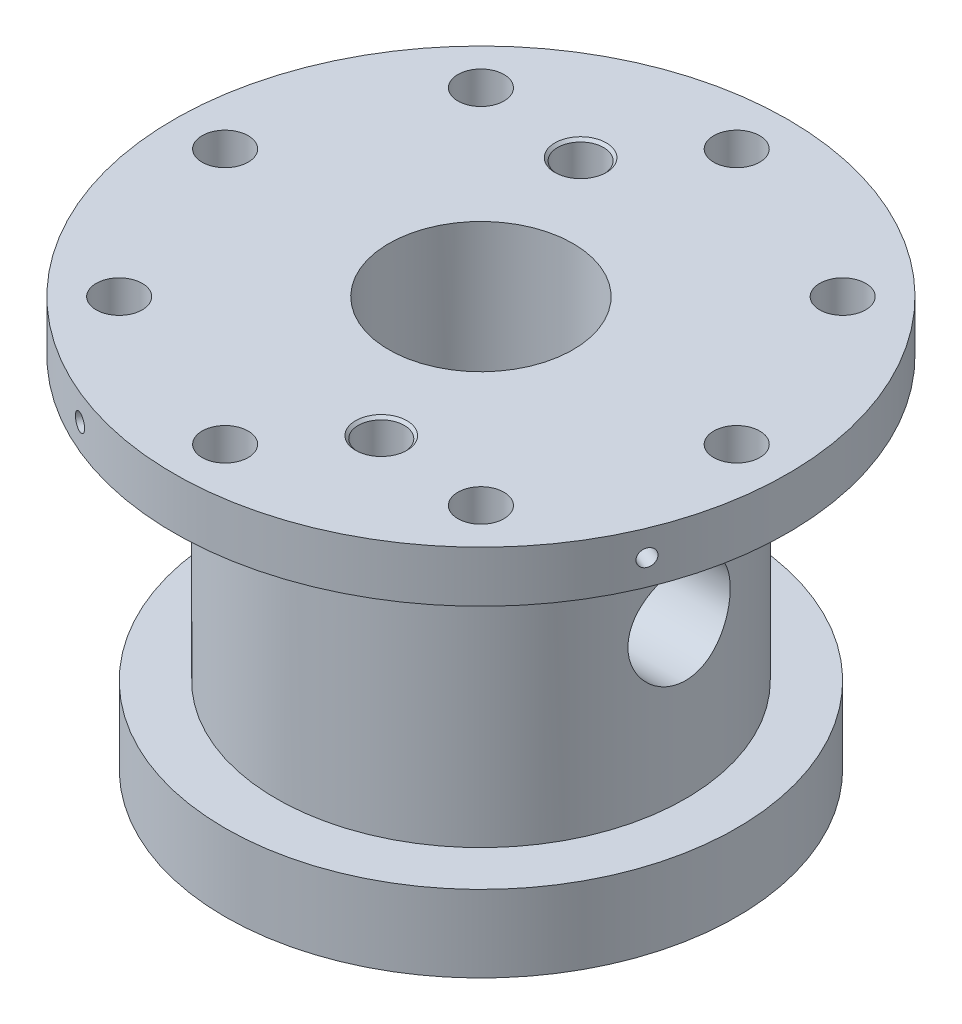
from build123d import *

# Parameters (mm, degrees)
SKETCH_2_R               = 4.5
CUT_EXTRUDE_1_DEPTH      = 10
PATTERN_CIRCULAR_1_COUNT = 8
EXTRUDE_START            = 10
SKETCH_3_R               = 40
EXTRUDE_1_DEPTH          = 10
SKETCH_7_R               = 18
EXTRUDE_2_DEPTH          = 10
SKETCH_5_W               = 5
SKETCH_5_H               = 30
CUT_EXTRUDE_2_DEPTH      = 15
PATTERN_CIRCULAR_3_COUNT = 3
PATTERN_CIRCULAR_4_COUNT = 4
EXTRUDE_3_DEPTH          = 10
EXTRUDE_3_DEPTH_BACK     = 5
SKETCH_11_R              = 50
SKETCH_11_W              = 5
SKETCH_11_H              = 30
M10X1_0_1_D              = 9
M10X1_0_1_DEPTH          = 23
M10X1_0_1_CSINK_D        = 10.05
M10X1_0_1_CSINK_ANGLE    = 90
M10X1_0_1_TIP            = 2.703872786
SKETCH_16_R              = 10
CUT_EXTRUDE_3_DEPTH      = 65


with BuildPart() as part:
    # 草图1 → 旋转1 (revolve)
    with BuildSketch(Plane.XY, mode=Mode.PRIVATE) as revolve_1_sk:
        Polygon((18, 60), (60, 60), (60, 50), (40, 50), (40, 0), (18, 0), align=None)
    revolve(revolve_1_sk.sketch.rotate(Axis((0, 0, 0), (0, 1, 0)), 90), axis=Axis((0, 0, 0), (0, 1, 0)))

    # 草图2 → 切除-拉伸1 (cut)
    with BuildSketch(Plane(origin=(0, 60, 0), x_dir=(1, 0, 0), z_dir=(0, 1, 0))):
        with Locations(Location((0, 50, 0), (0, 0, 270))):
            Circle(SKETCH_2_R)
    cut_extrude_1 = extrude(amount=-CUT_EXTRUDE_1_DEPTH, mode=Mode.SUBTRACT)

    # 阵列(圆周)1: 切除-拉伸1 ×8 about axis
    pattern_circular_1_axis = Axis((0, 0, 0), (0, 1, 0))
    for i in range(1, PATTERN_CIRCULAR_1_COUNT):
        add(cut_extrude_1.rotate(pattern_circular_1_axis, i * 360 / PATTERN_CIRCULAR_1_COUNT), mode=Mode.SUBTRACT)

    # 草图3 → 凸台-拉伸1 (add)
    with BuildSketch(Plane.XZ.offset(EXTRUDE_START)):
        with Locations(Location((0, 0, 0), (0, 0, 270))):
            Circle(SKETCH_3_R)
    extrude(amount=-EXTRUDE_1_DEPTH)

    # 草图7 → 凸台-拉伸2 (add)
    with BuildSketch(Plane(origin=(0, 0, 0), x_dir=(1, 0, 0), z_dir=(0, 1, 0)).offset(EXTRUDE_START)):
        with Locations(Location((0, 0, 0), (0, 0, 90))):
            Circle(SKETCH_7_R)
    extrude(amount=-EXTRUDE_2_DEPTH)

    # 草图5 → 切除-拉伸2 (cut)
    with BuildSketch(Plane.XZ.offset(10)):
        with Locations((0, 22)):
            Rectangle(SKETCH_5_W, SKETCH_5_H)
    cut_extrude_2 = extrude(amount=-CUT_EXTRUDE_2_DEPTH, mode=Mode.SUBTRACT)

    # 阵列(圆周)3: 切除-拉伸2 ×3 about axis
    pattern_circular_3_axis = Axis((0, 0, 0), (0, 1, 0))
    for i in range(1, PATTERN_CIRCULAR_3_COUNT):
        add(cut_extrude_2.rotate(pattern_circular_3_axis, i * 360 / PATTERN_CIRCULAR_3_COUNT), mode=Mode.SUBTRACT)

    # 草图10 → M4x0.7 螺纹孔1 (revolve, cut)
    with BuildSketch(Plane(origin=(22.961005942, 55, -55.432771951), x_dir=(-0.9238795325112892, 0, -0.3826834323650839), z_dir=(0, 1, 0))):
        Polygon((0, 0), (0, 11.091420021), (1.65, 10.1), (1.65, 0), align=None)
    m4x0_7_1 = revolve(axis=Axis((25.391045737, 55, -61.299406982), (-0.3826834323650839, 0, 0.9238795325112892)), mode=Mode.SUBTRACT)

    # 阵列(圆周)4: M4x0.7 螺纹孔1 ×4 about axis
    pattern_circular_4_axis = Axis((0, 0, 0), (0, -1, 0))
    for i in range(1, PATTERN_CIRCULAR_4_COUNT):
        add(m4x0_7_1.rotate(pattern_circular_4_axis, i * 360 / PATTERN_CIRCULAR_4_COUNT), mode=Mode.SUBTRACT)

    # 草图11 → 凸台-拉伸3 (add, two sides: drawn at the far end of the back side and taken through both)
    with BuildSketch(Plane.XZ.offset(10).offset(-EXTRUDE_3_DEPTH_BACK)):
        with Locations(Location((0, 0, 0), (0, 0, 270))):
            Circle(SKETCH_11_R)
        with Locations((0, 22)):
            Rectangle(SKETCH_11_W, SKETCH_11_H, mode=Mode.SUBTRACT)
        Polygon((-4.812177826, -5.665063509), (-30.79293994, -20.665063509), (-33.29293994, -16.334936491), (-7.312177826, -1.334936491), align=None, mode=Mode.SUBTRACT)
        Polygon((7.312177826, -1.334936491), (33.29293994, -16.334936491), (30.79293994, -20.665063509), (4.812177826, -5.665063509), align=None, mode=Mode.SUBTRACT)
    extrude(amount=EXTRUDE_3_DEPTH + EXTRUDE_3_DEPTH_BACK)

    # M10x1.0 螺纹孔1
    with Locations(Plane(origin=(-13.776603565, 60, -33.25966317), x_dir=(0, 0, 1), z_dir=(0, 1, 0))):
        with Locations((0, 0), (66.51932634, 27.55320713)):
            CounterSinkHole(M10X1_0_1_D / 2, M10X1_0_1_CSINK_D / 2, depth=M10X1_0_1_DEPTH, counter_sink_angle=M10X1_0_1_CSINK_ANGLE)
            with Locations((0, 0, -(M10X1_0_1_DEPTH + M10X1_0_1_TIP / 2))):  # 118° drill point
                Cone(0, M10X1_0_1_D / 2, M10X1_0_1_TIP, mode=Mode.SUBTRACT)

    # 草图16 → 切除-拉伸3 (cut, symmetric)
    with BuildSketch(Plane(origin=(0, 0, 0), x_dir=(0, 0, -1), z_dir=(1, 0, 0))):
        with Locations((0, 25)):
            Circle(SKETCH_16_R)
    extrude(amount=CUT_EXTRUDE_3_DEPTH, both=True, mode=Mode.SUBTRACT)


solid = part.part
